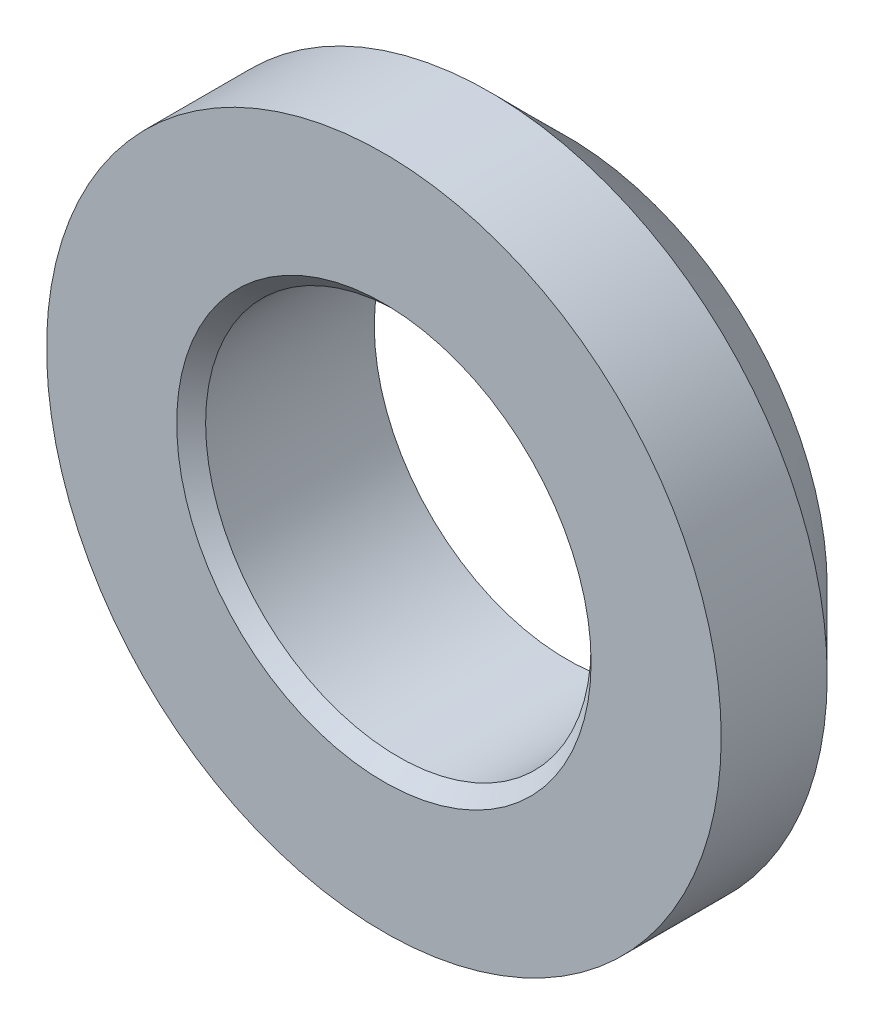
from build123d import *

# Parameters (mm, degrees)
SKETCH_1_R      = 35
SKETCH_1_R_2    = 20
EXTRUDE_1_DEPTH = 19
CHAMFER_1_SIZE  = 8
CHAMFER_2_SIZE  = 1.5


with BuildPart() as part:
    # 草图1 → 凸台-拉伸1 (new body)
    with BuildSketch(Plane.XY):
        Circle(SKETCH_1_R)
        Circle(SKETCH_1_R_2, mode=Mode.SUBTRACT)
    extrude(amount=EXTRUDE_1_DEPTH)

    # 倒角1
    chamfer_1_edges = [part.edges().sort_by_distance(p)[0] for p in [
        (-35, 0, 0),
    ]]
    chamfer(chamfer_1_edges, length=CHAMFER_1_SIZE)

    # 倒角2
    chamfer_2_edges = [part.edges().sort_by_distance(p)[0] for p in [
        (-20, 0, 19),
    ]]
    chamfer(chamfer_2_edges, length=CHAMFER_2_SIZE)


solid = part.part
